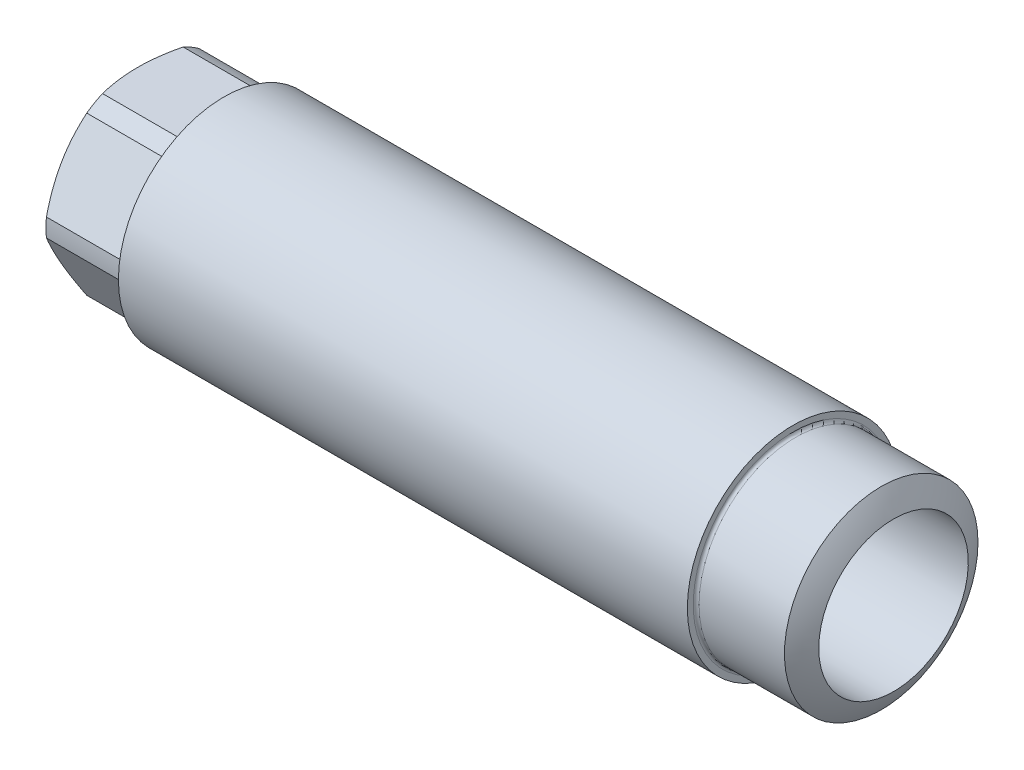
from build123d import *

# Parameters (mm, degrees)
SKETCH1_R          = 18
EXTRUDE1_DEPTH     = 132
SKETCH2_R          = 12.75
CUT_EXTRUDE1_DEPTH = 135.432139014
SKETCH3_R          = 18
SKETCH3_R_2        = 16.5
CUT_EXTRUDE2_DEPTH = 15
CUT_EXTRUDE3_START = -20
SKETCH4_R          = 18
SKETCH4_R_2        = 16.5
CUT_EXTRUDE3_DEPTH = 20
FILLET1_R          = 0.5
SKETCH6_R          = 25
CUT_EXTRUDE4_DEPTH = 14


with BuildPart() as part:
    # Sketch1 → Extrude1 (new body)
    with BuildSketch(Plane(origin=(0, 0, 0), x_dir=(0, 0, -1), z_dir=(1, 0, 0))):
        Circle(SKETCH1_R)
    extrude(amount=EXTRUDE1_DEPTH)

    # Sketch2 → Cut-Extrude1 (cut, through all)
    with BuildSketch(Plane.ZY):
        Circle(SKETCH2_R)
    extrude(amount=-CUT_EXTRUDE1_DEPTH, mode=Mode.SUBTRACT)

    # Sketch3 → Cut-Extrude2 (cut)
    with BuildSketch(Plane.ZY):
        Circle(SKETCH3_R)
        Circle(SKETCH3_R_2, mode=Mode.SUBTRACT)
    extrude(amount=-CUT_EXTRUDE2_DEPTH, mode=Mode.SUBTRACT)

    # Sketch4 → Cut-Extrude3 (cut)
    with BuildSketch(Plane(origin=(132, 0, 0), x_dir=(0, 0, -1), z_dir=(1, 0, 0)).offset(CUT_EXTRUDE3_START)):
        with Locations(Location((0, 0, 0), (0, 0, 180))):
            Circle(SKETCH4_R)
        with Locations(Location((0, 0, 0), (0, 0, 180))):
            Circle(SKETCH4_R_2, mode=Mode.SUBTRACT)
    extrude(amount=CUT_EXTRUDE3_DEPTH, mode=Mode.SUBTRACT)

    # Fillet1
    fillet1_edges = [part.edges().sort_by_distance(p)[0] for p in [
        (15, 0, -16.5),
        (112, 0, -16.5),
    ]]
    fillet(fillet1_edges, radius=FILLET1_R)

    # Sketch5 → Cut-Revolve1 (revolve, cut)
    with BuildSketch(Plane.XY, mode=Mode.PRIVATE) as cut_revolve1_sk:
        with BuildLine():
            Line((119.041447752, -42.253356684), (137.021599533, -42.253356684))
            Line((137.021599533, -42.253356684), (137.021599533, 0))
            Line((137.021599533, 0), (132, 0))
            ThreePointArc((132, 0), (128.56354111, -13.941961258), (119.041447752, -24.689857401))
            Line((119.041447752, -24.689857401), (119.041447752, -42.253356684))
        make_face()
    revolve(cut_revolve1_sk.sketch.rotate(Axis((132, 0, 0), (-1, 0, 0)), 180), axis=Axis((132, 0, 0), (-1, 0, 0)), mode=Mode.SUBTRACT)

    # Sketch6 → Cut-Extrude4 (cut)
    with BuildSketch(Plane.ZY):
        Circle(SKETCH6_R)
        Polygon((-8.660254038, -15), (8.660254038, -15), (17.320508076, 0), (8.660254038, 15), (-8.660254038, 15), (-17.320508076, 0), align=None, mode=Mode.SUBTRACT)
    extrude(amount=-CUT_EXTRUDE4_DEPTH, mode=Mode.SUBTRACT)

    # Sketch7 → Cut-Revolve2 (revolve, cut)
    with BuildSketch(Plane.XY, mode=Mode.PRIVATE) as cut_revolve2_sk:
        Polygon((0, -14.5), (0, -24.5), (5.773502692, -24.5), align=None)
    revolve(cut_revolve2_sk.sketch.rotate(Axis((15, 0, 0), (-1, 0, 0)), 270), axis=Axis((15, 0, 0), (-1, 0, 0)), mode=Mode.SUBTRACT)


solid = part.part
